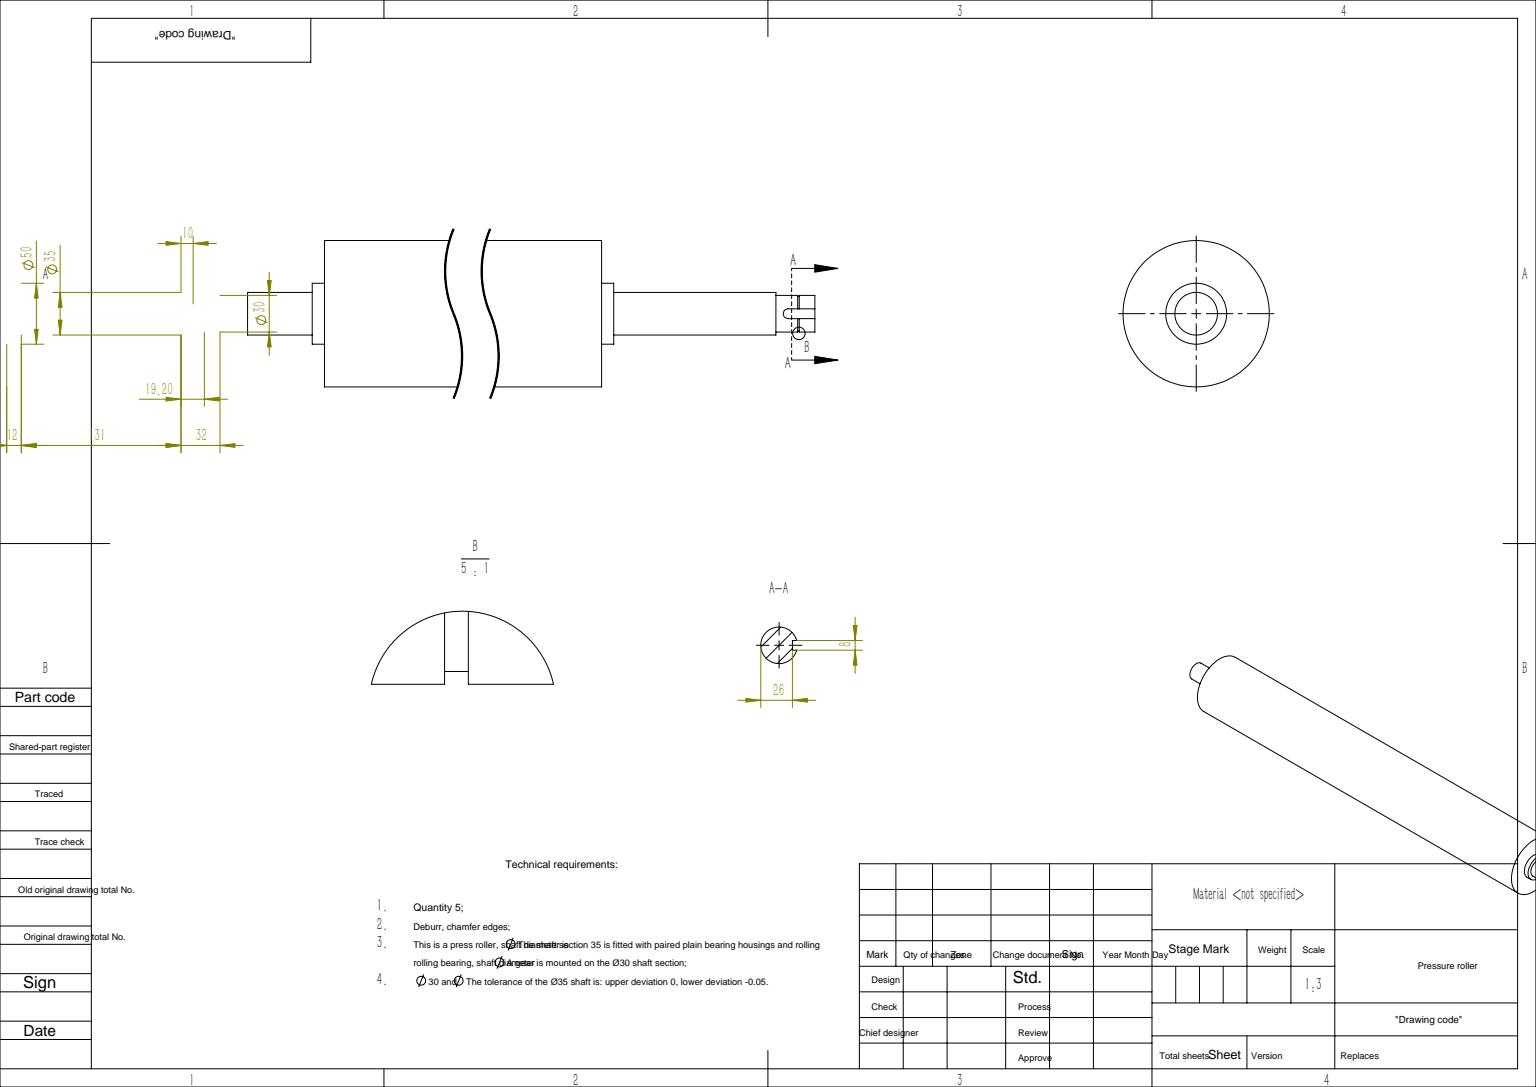
SolidWorks part; units mm, degrees
ref_plane "前视基准面" through (0, 0, 0) normal (0, 0, 1) x (1, 0, 0)
ref_plane "上视基准面" through (0, 0, 0) normal (0, 1, 0) x (1, 0, 0)
ref_plane "右视基准面" through (0, 0, 0) normal (1, 0, 0) x (0, 0, -1)
sketch "草图1" plane through (0, 0, 0) normal (0, 0, 1) x (1, 0, 0)
  line L0 (0, 0) -> (0, 17.5)
  line L1 (0, 17.5) -> (53, 17.5)
  line L2 (53, 17.5) -> (53, 25)
  line L3 (53, 25) -> (63, 25)
  line L4 (63, 25) -> (63, 60)
  line L5 (63, 60) -> (913, 60)
  line L6 (913, 60) -> (913, 25)
  line L7 (913, 25) -> (923, 25)
  line L8 (923, 25) -> (923, 17.5)
  line L9 (923, 17.5) -> (1056, 17.5)
  line L10 (1056, 17.5) -> (1056, 15)
  line L11 (1056, 15) -> (1088, 15)
  line L12 (1088, 15) -> (1088, 0)
  line L13 (1088, 0) -> (0, 0)
  dimension "D1" = 53
  dimension "D2" = 10
  dimension "D3" = 850
  dimension "D4" = 17.5
  dimension "D5" = 25
  dimension "D6" = 60
  dimension "D7" = 25
  dimension "D8" = 10
  dimension "D9" = 17.5
  dimension "D10" = 133
  dimension "D11" = 32
  dimension "D12" = 15
revolve "旋转1" add sketch "草图1" angle 360 about L13
ref_plane "基准面1" through (0, 15, 0) normal (0, 1, 0) x (1, 0, 0)
sketch "草图2" plane through (0, 15, 0) normal (0, 1, 0) x (1, 0, 0)
  line L0 (1056, 0) -> (1088, 0) construction
  line L1 (1056, -15) -> (1056, 15) construction
  line L2 (1088, -15) -> (1088, 15) construction
  line L3 (1066, 4) -> (1098, 4)
  line L4 (1098, 4) -> (1098, -4)
  line L5 (1098, -4) -> (1066, -4)
  line L6 (1056, -17.5) -> (1056, 17.5) construction
  arc A0 (1066, 4) -> (1066, -4) centre (1066, 0) ccw
  dimension "D1" = 4
  dimension "D2" = 10
  dimension "D3" = 10
extrude "切除-拉伸1" cut sketch "草图2" against normal blind 4
ref_plane "基准面2" through (1075.2, 0, 0) normal (1, 0, 0) x (0, 0, -1)
sketch "草图3" plane through (1075.2, 0, 0) normal (1, 0, 0) x (0, 0, -1)
  circle A0 centre (0, 0) radius 15
  arc A1 (-4, 14.4568) -> (4, 14.4568) centre (0, 0) ccw construction
  circle A2 centre (0, 0) radius 14.3
  dimension "D1" = 28.6
extrude "切除-拉伸2" cut sketch "草图3" against normal blind 1.3
